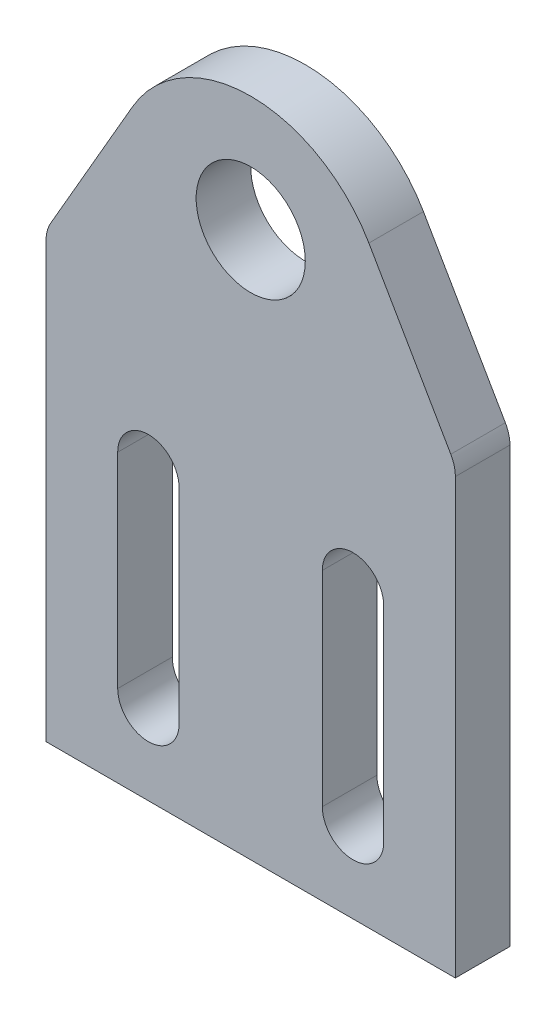
SolidWorks part; units mm, degrees
material "Q235"
ref_plane "Front" through (0, 0, 0) normal (0, 0, 1) x (1, 0, 0)
ref_plane "Top" through (0, 0, 0) normal (0, 1, 0) x (1, 0, 0)
ref_plane "Right" through (0, 0, 0) normal (1, 0, 0) x (0, 0, -1)
sketch "Sketch2" plane through (0, 0, 0) normal (0, 0, 1) x (1, 0, 0)
  line L0 (0, 0) -> (0, 65)
  line L1 (0, 65) -> (12.6795, 86.9615)
  line L2 (47.3205, 86.9615) -> (60, 65)
  line L3 (60, 65) -> (60, 0)
  line L4 (60, 0) -> (0, 0)
  line L5 (30, 0) -> (30, 65) construction
  arc A0 (12.6795, 86.9615) -> (47.3205, 86.9615) centre (30, 76.9615) cw
  dimension "D1" = 60
  dimension "D4" = 20
  dimension "D2" = 65
  dimension "D3" = 60
extrude "Boss-Extrude1" add sketch "Sketch2" along normal blind 8
sketch "Sketch3" plane through (0, 0, 8) normal (0, 0, 1) x (1, 0, 0)
  line L0 (30, 0) -> (30, 80) construction
  line L1 (0, 0) -> (60, 0) construction
  circle A0 centre (30, 80) radius 8
  dimension "D1" = 16
  dimension "D2" = 80
extrude "Cut-Extrude1" cut sketch "Sketch3" against normal blind 8
sketch "Sketch4" plane through (0, 0, 8) normal (0, 0, 1) x (1, 0, 0)
  line L0 (15, 12) -> (15, 42) construction
  line L1 (10.5, 12) -> (10.5, 42)
  line L2 (19.5, 12) -> (19.5, 42)
  line L3 (30, 0) -> (30, 17.85) construction
  line L4 (0, 0) -> (60, 0) construction
  line L5 (45, 12) -> (45, 42) construction
  line L6 (49.5, 12) -> (49.5, 42)
  line L7 (40.5, 12) -> (40.5, 42)
  arc A0 (10.5, 12) -> (19.5, 12) centre (15, 12) ccw
  arc A1 (19.5, 42) -> (10.5, 42) centre (15, 42) ccw
  arc A2 (49.5, 12) -> (40.5, 12) centre (45, 12) cw
  arc A3 (40.5, 42) -> (49.5, 42) centre (45, 42) cw
  point P2 (15, 27)
  point P13 (45, 27)
  dimension "D2" = 30
  dimension "D4" = 12
  dimension "D1" = 9
  dimension "D3" = 30
extrude "Cut-Extrude2" cut sketch "Sketch4" against normal through all
fillet "Fillet1" radius 5 2 edges at (60, 65, 4) (0, 65, 4)
sketch "Sketch5" plane through (0, 0, 8) normal (0, 0, 1) x (1, 0, 0)
  circle A0 centre (30, 80) radius 25
  dimension "D1" = 50
